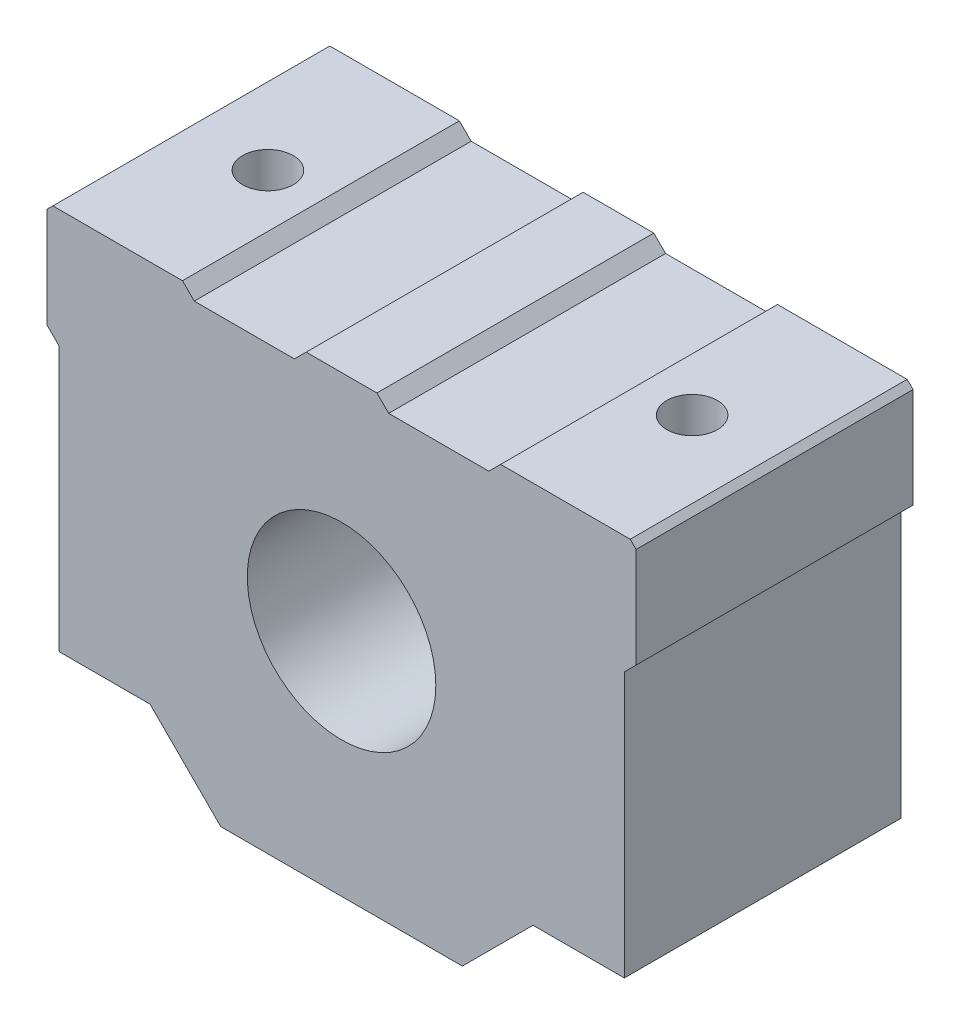
SolidWorks part; units mm, degrees
ref_plane "前视基准面" through (0, 0, 0) normal (0, 0, 1) x (1, 0, 0)
ref_plane "上视基准面" through (0, 0, 0) normal (0, 1, 0) x (1, 0, 0)
ref_plane "右视基准面" through (0, 0, 0) normal (1, 0, 0) x (0, 0, -1)
sketch "草图1" plane through (0, 0, 0) normal (0, 0, 1) x (1, 0, 0)
  line L0 (-10.25, -19.5) -> (10.25, -19.5)
  line L1 (16.25, -13.5) -> (10.25, -19.5)
  line L2 (16.25, -13.5) -> (24, -13.5)
  line L3 (24, -13.5) -> (24, 9)
  line L4 (24, 9) -> (25, 10)
  line L5 (25, 10) -> (25, 18.5)
  line L6 (24.5, 19) -> (13.5, 19)
  line L7 (13.5, 19) -> (12.5, 18)
  line L8 (12.5, 18) -> (4, 18)
  line L9 (4, 18) -> (3, 19)
  line L10 (3, 19) -> (-3, 19)
  line L11 (-3, 19) -> (-4, 18)
  line L12 (-4, 18) -> (-12.5, 18)
  line L13 (-12.5, 18) -> (-13.5, 19)
  line L14 (-13.5, 19) -> (-24.5, 19)
  line L15 (-25, 18.5) -> (-25, 10)
  line L16 (-25, 10) -> (-24, 9)
  line L17 (-24, 9) -> (-24, -13.5)
  line L18 (-24, -13.5) -> (-16.25, -13.5)
  line L19 (-16.25, -13.5) -> (-10.25, -19.5)
  line L20 (-24.5, 19) -> (-25, 18.5)
  line L21 (25, 18.5) -> (24.5, 19)
  line L22 (0, 19) -> (0, -19.5) construction
  circle A0 centre (0, 0) radius 8
  point P10 (25, 19)
  point P19 (-25, 19)
  dimension "D1" = 16
  dimension "D2" = 0.5
  dimension "D3" = 45
  dimension "D4" = 0.5
  dimension "D5" = 45
  dimension "D6" = 32.5
  dimension "D7" = 135
  dimension "D8" = 135
  dimension "D9" = 32.5
  dimension "D10" = 1
  dimension "D11" = 135
  dimension "D12" = 135
  dimension "D13" = 38.5
  dimension "D14" = 9
  dimension "D15" = 6
  dimension "D16" = 27
  dimension "D17" = 50
  dimension "D18" = 1
  dimension "D19" = 19
  dimension "D20" = 135
  dimension "D21" = 135
  dimension "D22" = 135
  dimension "D23" = 135
extrude "凸台-拉伸1" add sketch "草图1" along normal blind 23.5
sketch "草图2" plane through (0, 19, 0) normal (0, 1, 0) x (1, 0, 0)
  circle A0 centre (-18, -11.75) radius 2.15
  circle A1 centre (18, -11.75) radius 2.15
  dimension "D3" = 4.3
  dimension "D1" = 11.75
  dimension "D2" = 36
  dimension "D4" = 18
extrude "切除-拉伸1" cut sketch "草图2" against normal through all
cosmetic thread "装饰螺纹线1" parameters "D1"=12, "D2"=5
cosmetic thread "装饰螺纹线2" parameters "D1"=12, "D2"=5
